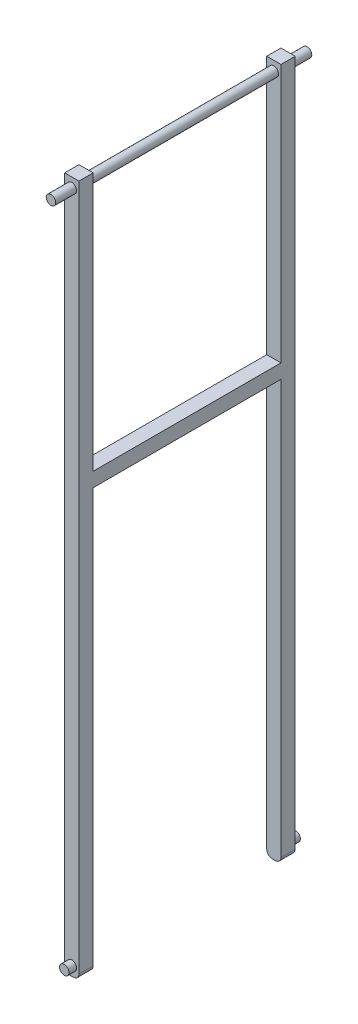
from build123d import *

# Parameters (mm, degrees)
SKETCH1_W                = 15
SKETCH1_H                = 15
BOSS_EXTRUDE1_DEPTH      = 730
SKETCH2_R                = 5
BOSS_EXTRUDE2_DEPTH      = 8
SKETCH4_W                = 15
SKETCH4_H                = 15
BOSS_EXTRUDE3_DEPTH      = 198
SKETCH5_W                = 15
SKETCH5_H                = 730
BOSS_EXTRUDE4_DEPTH      = 15
BOSS_EXTRUDE5_START      = 8
SKETCH6_R                = 5
BOSS_EXTRUDE5_DEPTH      = 8
FILLET1_R                = 6
BOSS_EXTRUDE6_DEPTH      = 20
BOSS_EXTRUDE6_DEPTH_BACK = 250
SKETCH7_R                = 5


with BuildPart() as part:
    # Sketch1 → Boss-Extrude1 (new body)
    with BuildSketch(Plane(origin=(0, 0, 0), x_dir=(1, 0, 0), z_dir=(0, 1, 0))):
        Rectangle(SKETCH1_W, SKETCH1_H)
    extrude(amount=BOSS_EXTRUDE1_DEPTH)

    # Sketch2 → Boss-Extrude2 (add)
    with BuildSketch(Plane(origin=(0, 0, -7.5), x_dir=(-1, 0, 0), z_dir=(0, 0, -1))):
        with Locations(Location((0, 10, 0), (0, 0, 180))):
            Circle(SKETCH2_R)
    extrude(amount=BOSS_EXTRUDE2_DEPTH)

    # Sketch4 → Boss-Extrude3 (add)
    with BuildSketch(Plane.XY.offset(7.5)):
        with Locations((0, 450)):
            Rectangle(SKETCH4_W, SKETCH4_H)
    extrude(amount=BOSS_EXTRUDE3_DEPTH)

    # Sketch5 → Boss-Extrude4 (add)
    with BuildSketch(Plane.XY.offset(205.5)):
        with Locations((0, 365)):
            Rectangle(SKETCH5_W, SKETCH5_H)
    extrude(amount=BOSS_EXTRUDE4_DEPTH)

    # Sketch6 → Boss-Extrude5 (add)
    with BuildSketch(Plane.XY.offset(220.5).offset(BOSS_EXTRUDE5_START)):
        with Locations((0, 10)):
            Circle(SKETCH6_R)
    extrude(amount=-BOSS_EXTRUDE5_DEPTH)

    # Fillet1
    fillet1_edges = [part.edges().sort_by_distance(p)[0] for p in [
        (7.5, 0, 213),
        (-7.5, 0, 213),
        (-7.5, 0, 0),
        (7.5, 0, 0),
    ]]
    fillet(fillet1_edges, radius=FILLET1_R)

    # Sketch7 → Boss-Extrude6 (add, two sides: drawn at the far end of the back side and taken through both)
    with BuildSketch(Plane(origin=(0, 0, -7.5), x_dir=(-1, 0, 0), z_dir=(0, 0, -1)).offset(-BOSS_EXTRUDE6_DEPTH_BACK)):
        with Locations(Location((0, 720, 0), (0, 0, 180))):
            Circle(SKETCH7_R)
    extrude(amount=BOSS_EXTRUDE6_DEPTH + BOSS_EXTRUDE6_DEPTH_BACK)


solid = part.part
